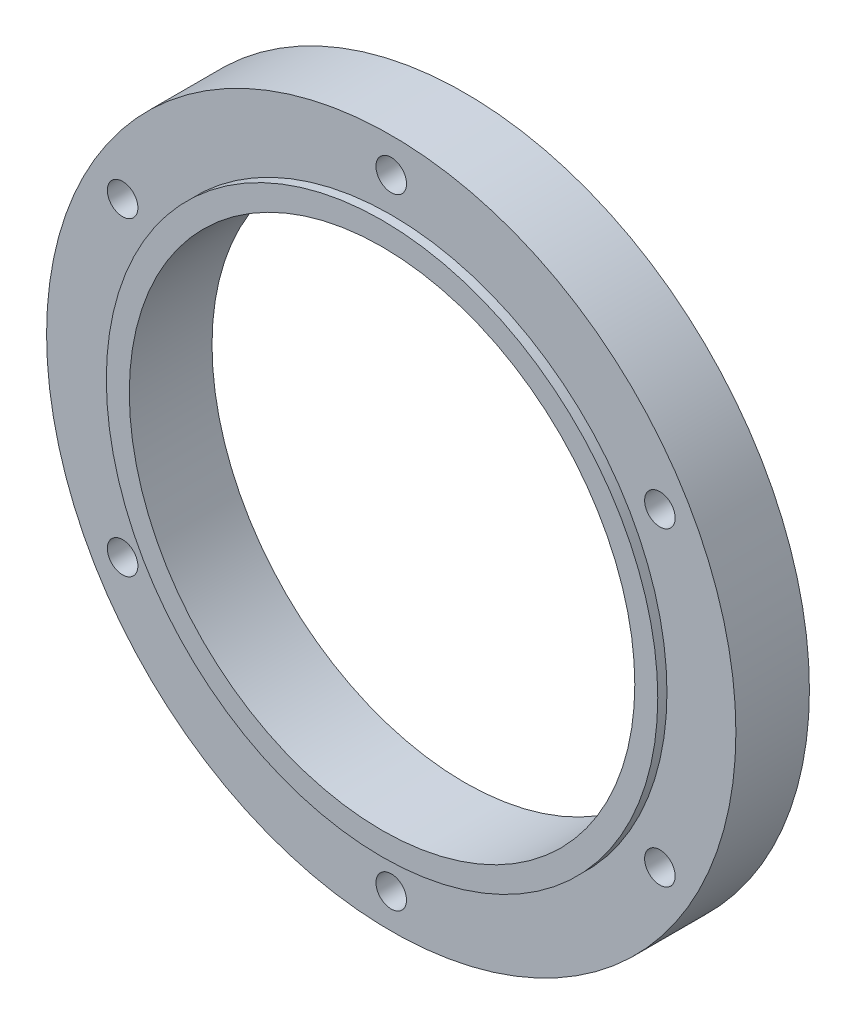
SolidWorks part; units mm, degrees
ref_plane "Front Plane" through (0, 0, 0) normal (0, 0, 1) x (1, 0, 0)
ref_plane "Top Plane" through (0, 0, 0) normal (0, 1, 0) x (1, 0, 0)
ref_plane "Right Plane" through (0, 0, 0) normal (1, 0, 0) x (0, 0, -1)
sketch "Sketch1" plane through (0, 0, 0) normal (0, 0, 1) x (1, 0, 0)
  circle A0 centre (0, 0) radius 55
  circle A1 centre (0, 0) radius 75
  circle A2 centre (0, 0) radius 67.5 construction
  circle A3 centre (0, 67.5) radius 3.325
  circle A4 centre (58.4567, 33.75) radius 3.325
  circle A5 centre (58.4567, -33.75) radius 3.325
  circle A6 centre (0, -67.5) radius 3.325
  circle A7 centre (-58.4567, -33.75) radius 3.325
  circle A8 centre (-58.4567, 33.75) radius 3.325
  dimension "D1" = 150
  dimension "D2" = 135
  dimension "D3" = 110
  dimension "D4" = 6.65
  dimension "D6" = 58.4567
  dimension "D7" = 67.5
  dimension "D5" = 6
extrude "Boss-Extrude1" add sketch "Sketch1" along normal blind 16
sketch "Sketch2" plane through (0, 0, 16) normal (0, 0, 1) x (1, 0, 0)
  circle A0 centre (0, 0) radius 55
  circle A1 centre (0, 0) radius 60
  dimension "D1" = 5
  dimension "D2" = 110
extrude "Boss-Extrude2" add sketch "Sketch2" along normal blind 2
